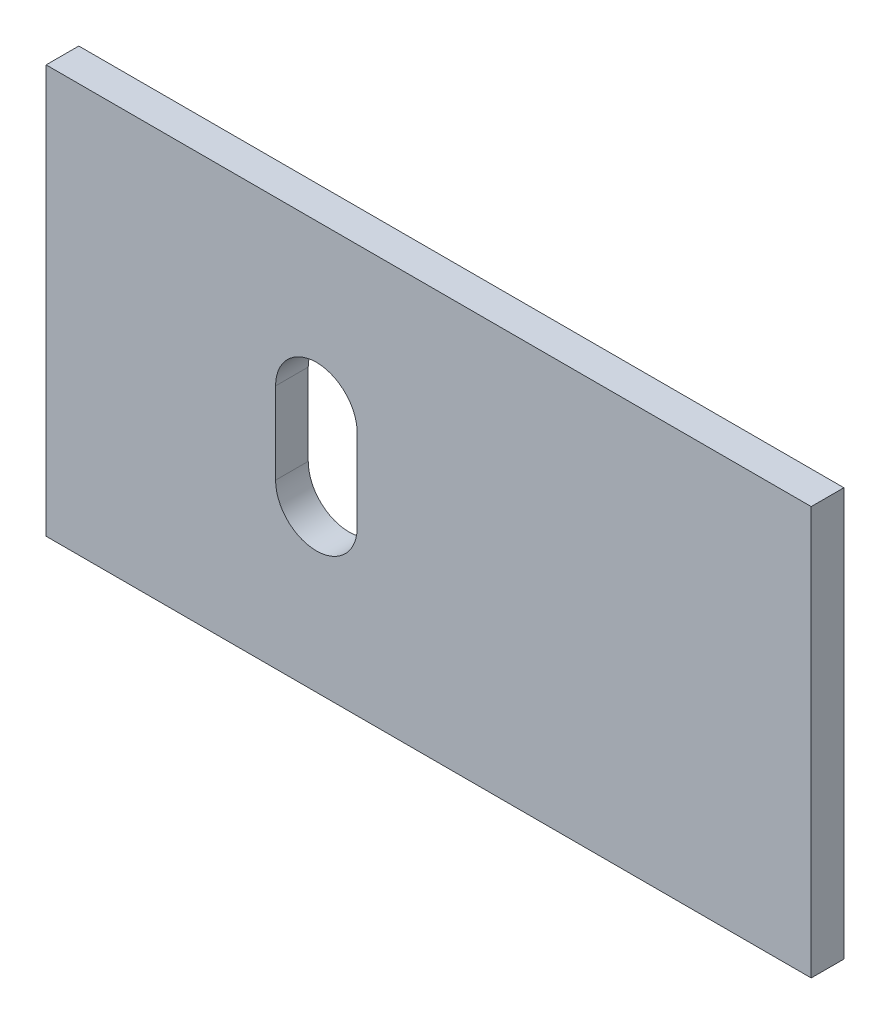
from build123d import *

# Parameters (mm, degrees)
BOSS_EXTRUDE1_DEPTH = 20


with BuildPart() as part:
    # Sketch1 → Boss-Extrude1 (new body)
    with BuildSketch(Plane.XY):
        Polygon((9106.725741881, 4668.311117452), (9575.225782872, 4668.311117452), (9575.225782872, 4418.311117452), (9106.725741967, 4418.311117452), align=None)
        with BuildLine():
            Line((9247.225783525, 4568.310529412), (9247.225783525, 4518.311318924))
            ThreePointArc((9247.225783525, 4518.311318924), (9272.225682554, 4493.311117122), (9297.225783432, 4518.311117075))
            Line((9297.225783432, 4518.311117075), (9297.225783432, 4568.311116981))
            ThreePointArc((9297.225783432, 4568.311116981), (9272.225489694, 4593.31082315), (9247.225783525, 4568.310529412))
        make_face(mode=Mode.SUBTRACT)
    extrude(amount=BOSS_EXTRUDE1_DEPTH)


solid = part.part
